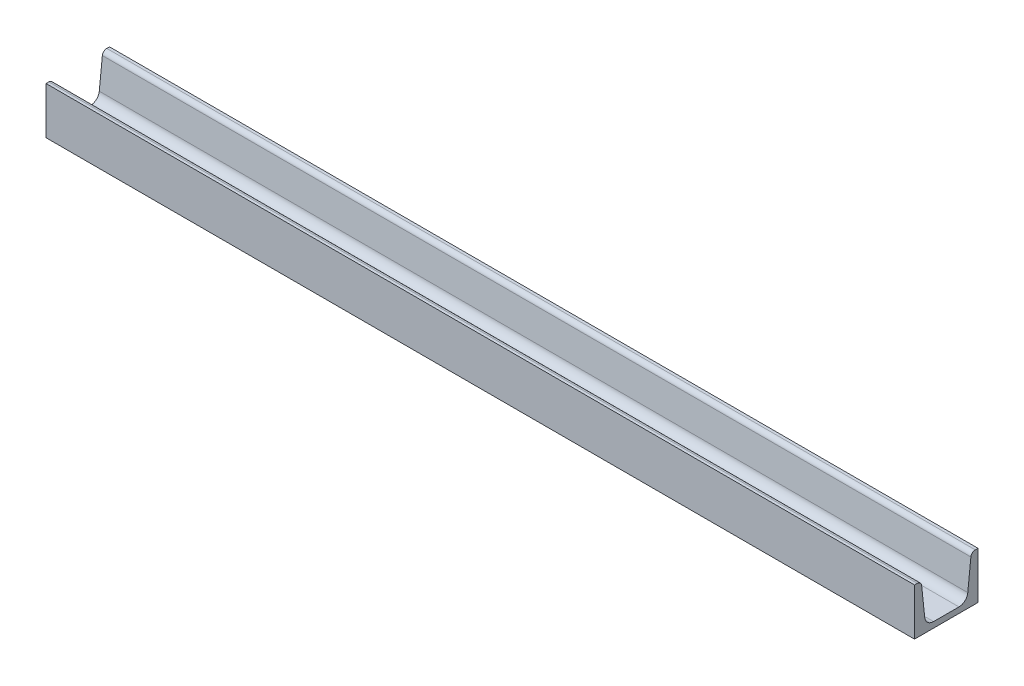
from build123d import *

# Parameters (mm, degrees)
GB_T_707_1988_HOT_ROLLED_CHANNEL_05_1_DEPTH = 684


with BuildPart() as part:
    # Sketch1 → GB/T 707-1988 hot-rolled channel 05(1) (new body)
    with BuildSketch(Plane.YZ.offset(-342)):
        with BuildLine():
            Line((37, 50), (0, 50))
            Line((0, 50), (0, 0))
            Line((0, 0), (37, 0))
            Line((37, 0), (37, 2.140642022))
            ThreePointArc((37, 2.140642022), (36.101006889, 4.482599144), (33.865849621, 5.621468656))
            Line((33.865849621, 5.621468656), (10.768300757, 8.049118866))
            ThreePointArc((10.768300757, 8.049118866), (6.297986222, 10.326857889), (4.5, 15.010772133))
            Line((4.5, 15.010772133), (4.5, 34.989227867))
            ThreePointArc((4.5, 34.989227867), (6.297986222, 39.673142111), (10.768300757, 41.950881134))
            Line((10.768300757, 41.950881134), (33.865849621, 44.378531344))
            ThreePointArc((33.865849621, 44.378531344), (36.101006889, 45.517400856), (37, 47.859357978))
            Line((37, 47.859357978), (37, 50))
        make_face()
    extrude(amount=GB_T_707_1988_HOT_ROLLED_CHANNEL_05_1_DEPTH)


solid = part.part
